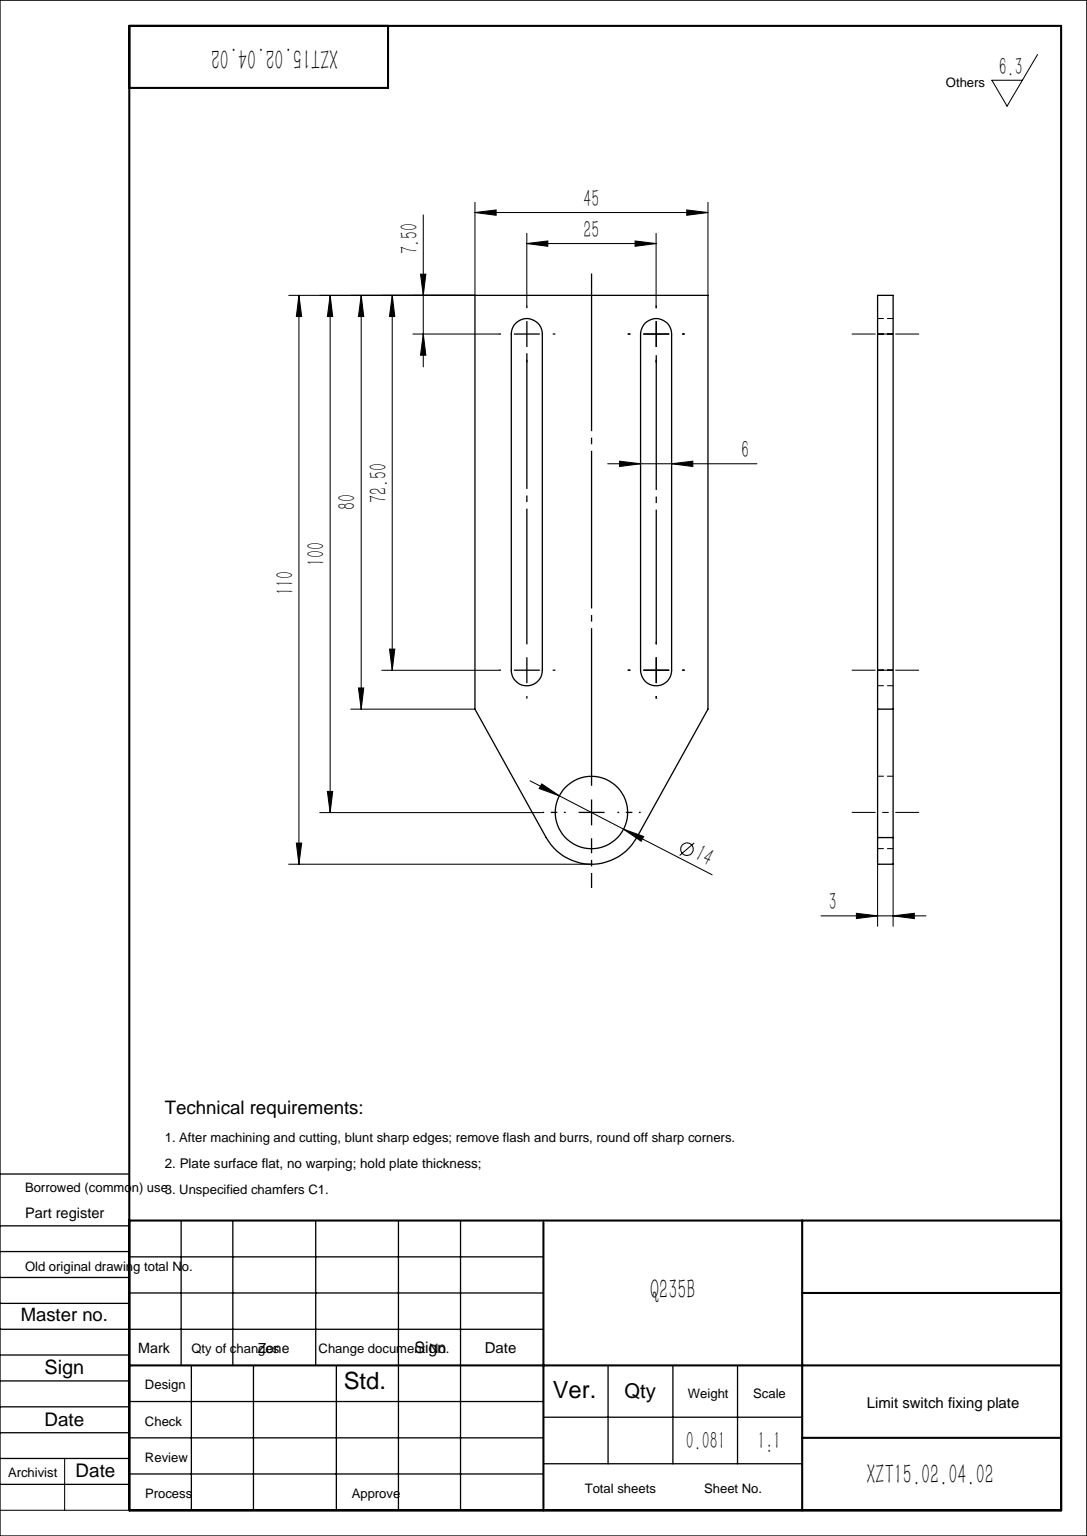
from build123d import *

# Parameters (mm, degrees)
SKETCH1_R           = 7
BOSS_EXTRUDE1_DEPTH = 3


with BuildPart() as part:
    # Sketch1 → Boss-Extrude1 (new body)
    with BuildSketch(Plane(origin=(0, 0, 0), x_dir=(1, 0, 0), z_dir=(0, 1, 0))):
        with BuildLine():
            Line((-22.5, 100), (22.5, 100))
            Line((22.5, 100), (22.5, 20))
            Line((22.5, 20), (8.749140244, -4.842782774))
            ThreePointArc((8.749140244, -4.842782774), (0, -10), (-8.749140244, -4.842782774))
            Line((-8.749140244, -4.842782774), (-22.5, 20))
            Line((-22.5, 20), (-22.5, 100))
        make_face()
        with Locations(Location((0, 0, 0), (0, 0, 270))):
            Circle(SKETCH1_R, mode=Mode.SUBTRACT)
        with BuildLine():
            Line((-15.5, 27.5), (-15.5, 92.5))
            ThreePointArc((-15.5, 92.5), (-12.5, 95.5), (-9.5, 92.5))
            Line((-9.5, 92.5), (-9.5, 27.5))
            ThreePointArc((-9.5, 27.5), (-12.5, 24.5), (-15.5, 27.5))
        make_face(mode=Mode.SUBTRACT)
        with BuildLine():
            Line((15.5, 27.5), (15.5, 92.5))
            ThreePointArc((15.5, 92.5), (12.5, 95.5), (9.5, 92.5))
            Line((9.5, 92.5), (9.5, 27.5))
            ThreePointArc((9.5, 27.5), (12.5, 24.5), (15.5, 27.5))
        make_face(mode=Mode.SUBTRACT)
    extrude(amount=BOSS_EXTRUDE1_DEPTH)


solid = part.part
